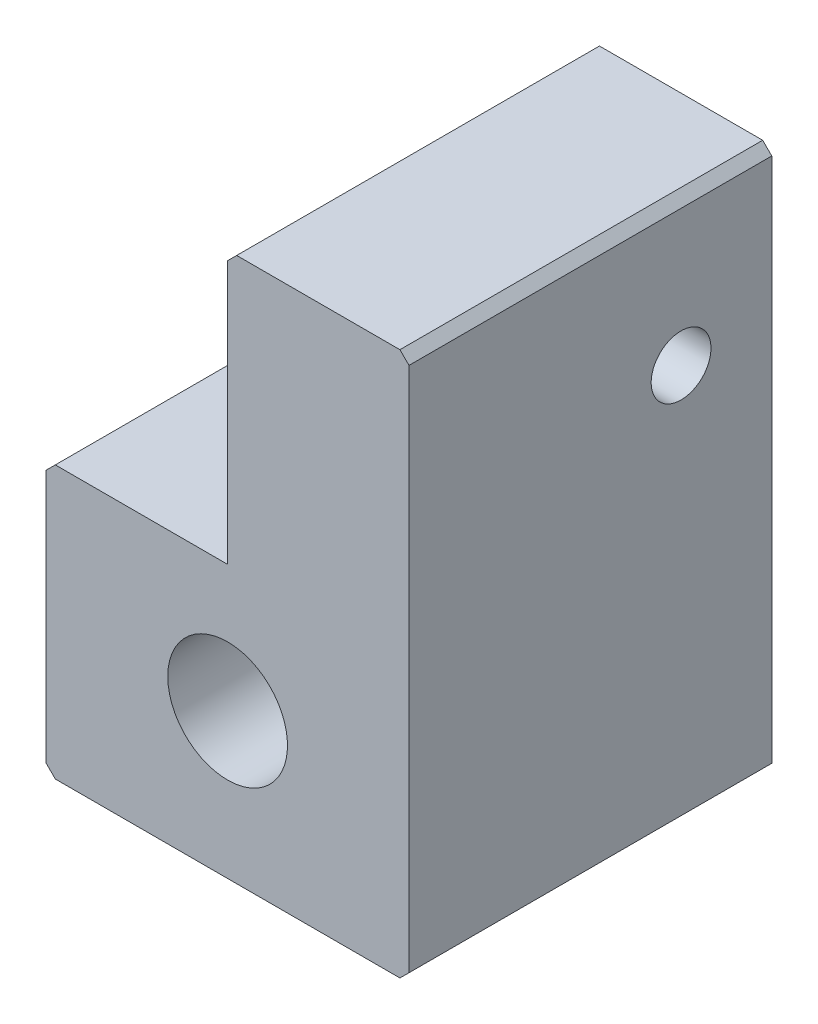
SolidWorks part; units mm, degrees
material "A6061"
ref_plane "前基準面" through (0, 0, 0) normal (0, 0, 1) x (1, 0, 0)
ref_plane "上基準面" through (0, 0, 0) normal (0, 1, 0) x (1, 0, 0)
ref_plane "右基準面" through (0, 0, 0) normal (1, 0, 0) x (0, 0, -1)
sketch "草图1" plane through (0, 0, 0) normal (0, 0, 1) x (1, 0, 0)
  line L1 (-10, 15) -> (10, 15)
  line L2 (-10, 15) -> (-10, -15)
  line L3 (-10, -15) -> (10, -15)
  line L4 (10, 15) -> (10, -15)
  line L5 (-10, 15) -> (10, -15) construction
  line L6 (-10, -15) -> (10, 15) construction
  point P0 (0, 0)
  dimension "D1" = 20
  dimension "D2" = 30
extrude "凸台-拉伸1" add sketch "草图1" along normal blind 20
hole_wizard "打孔尺寸根据内六角圆柱头螺钉的类型1" positions "草图3" profile "草图2" counterbore size "M6" standard "GB" end condition through all
sketch "草图3" plane through (3.1336, 10.9079, 0) normal (0, 0, 1) x (1, 0, 0)
  line L0 (-3.1336, -10.9079) -> (-3.1336, -25.1536) construction
  line L2 (-13.1336, -25.9079) -> (6.8664, -25.9079) construction
  point P0 (-3.1336, -17.9079)
  dimension "D1" = 8
sketch "草图2" plane through (0, -7, 0) normal (1, 0, 0) x (0, 1, 0)
  line L0 (0, 0) -> (0, 20)
  line L1 (0, 20) -> (3.3, 20)
  line L3 (3.3, 20) -> (3.3, 6.8)
  line L4 (3.3, 6.8) -> (5.5, 6.8)
  line L5 (5.5, 6.8) -> (5.5, 0)
  line L7 (5.5, 0) -> (0, 0)
  line L11 (0, -6.35) -> (0, 107.95) construction
  dimension "通孔孔直径" = 6.6
  dimension "通孔孔深度" = 20
  dimension "柱形沉头孔直径" = 11
  dimension "柱形沉头孔深度" = 6.8
sketch "草图4" plane through (0, 0, 20) normal (0, 0, 1) x (1, 0, 0)
  line L0 (-10, -15) -> (10, -15) construction
  line L1 (-10, 15) -> (0, 15)
  line L2 (-10, 15) -> (-10, 0)
  line L3 (-10, 0) -> (0, 0)
  line L4 (0, 15) -> (0, 0)
  dimension "D1" = 10
  dimension "D2" = 15
extrude "切除-拉伸1" cut sketch "草图4" against normal through all
hole_wizard "M4 螺纹孔1" positions "草图6" profile "草图5" tap size "M4" standard "GB" end condition through all
sketch "草图6" plane through (0, 0, 0) normal (-1, 0, 0) x (0, 0, 1)
  line L2 (0, 0) -> (20, 0) construction
  line L3 (20, 0) -> (20, 15) construction
  point P0 (5, 7)
  dimension "D1" = 15
  dimension "D2" = 7
sketch "草图5" plane through (0, 7, 5) normal (0, 1, 0) x (0, 0, 1)
  line L0 (0, 0) -> (0, 10)
  line L1 (0, 10) -> (1.65, 10)
  line L2 (1.65, 10) -> (1.65, 0)
  line L5 (1.65, 0) -> (0, 0)
  line L11 (0, -6.35) -> (0, 107.95) construction
  dimension "通孔螺纹孔钻头直径" = 3.3
  dimension "通孔螺纹孔钻头深度" = 10
cosmetic thread "孔螺蚊线1" parameters "D2"=4
chamfer "倒角1" distance 0.5 angle 45 5 edges at (10, 15, 10) (0, 15, 10) (-10, 0, 10) (-10, -15, 10) (10, -15, 10)
